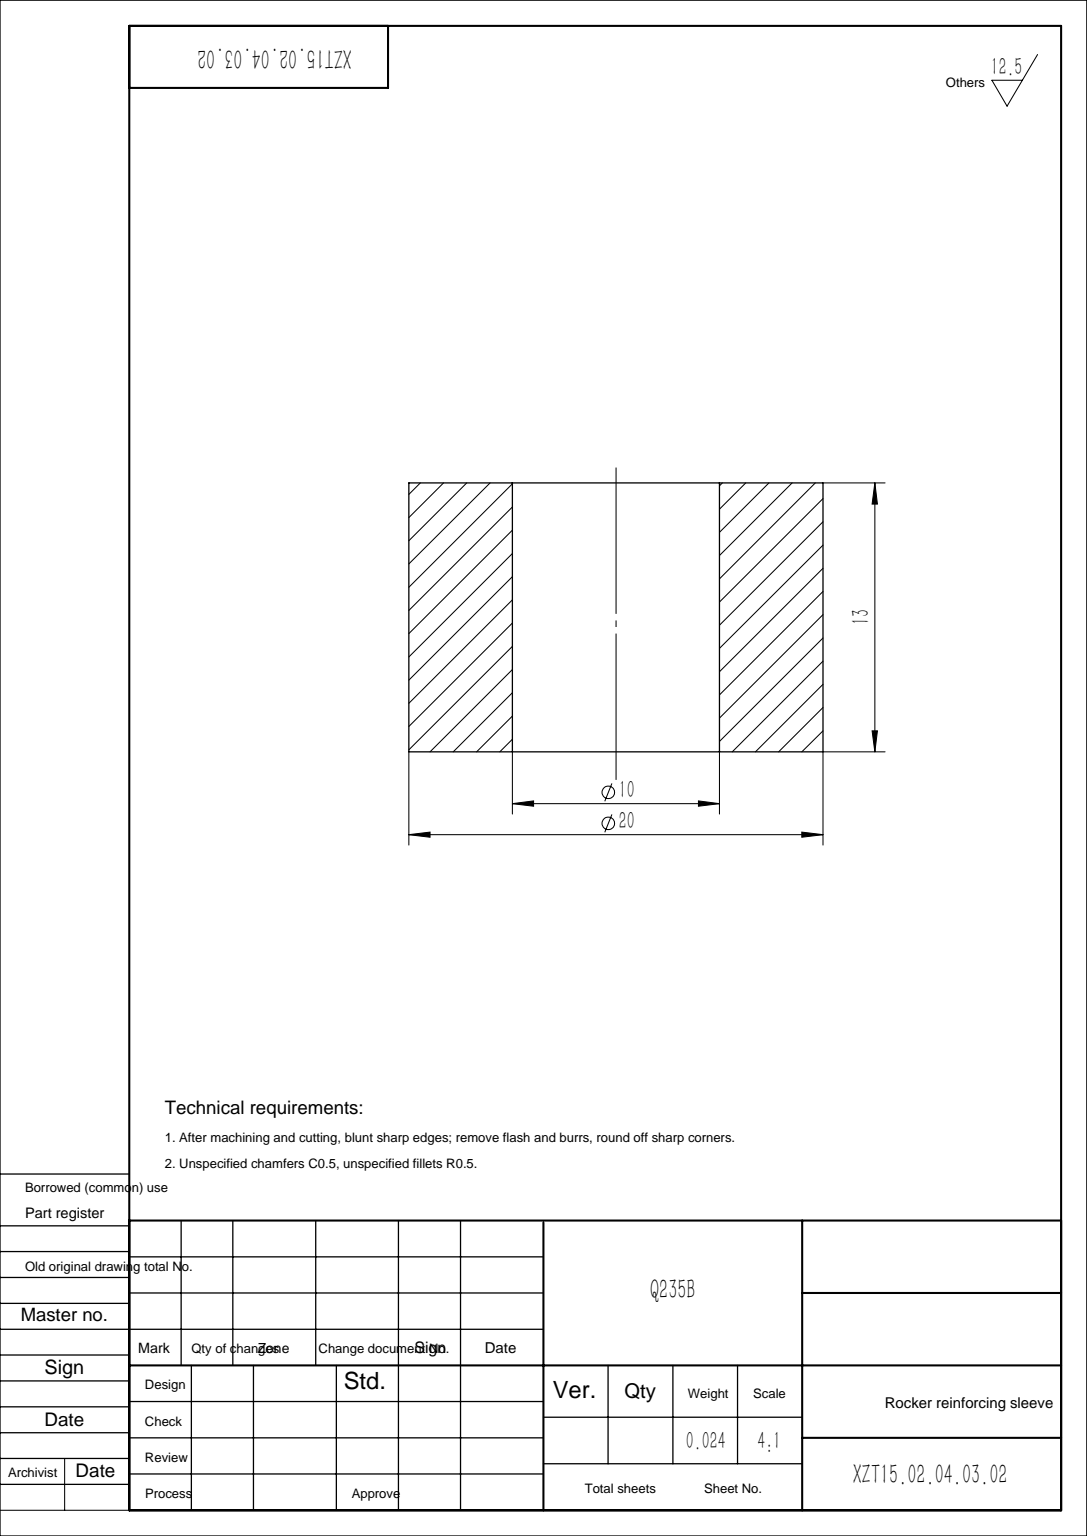
from build123d import *

# Parameters (mm, degrees)
SKETCH1_R           = 10
SKETCH1_R_2         = 5
BOSS_EXTRUDE1_DEPTH = 13


with BuildPart() as part:
    # Sketch1 → Boss-Extrude1 (new body)
    with BuildSketch(Plane(origin=(0, 0, 0), x_dir=(1, 0, 0), z_dir=(0, 1, 0))):
        with Locations(Location((0, 0, 0), (0, 0, 90))):
            Circle(SKETCH1_R)
        with Locations(Location((0, 0, 0), (0, 0, 90))):
            Circle(SKETCH1_R_2, mode=Mode.SUBTRACT)
    extrude(amount=BOSS_EXTRUDE1_DEPTH)


solid = part.part
